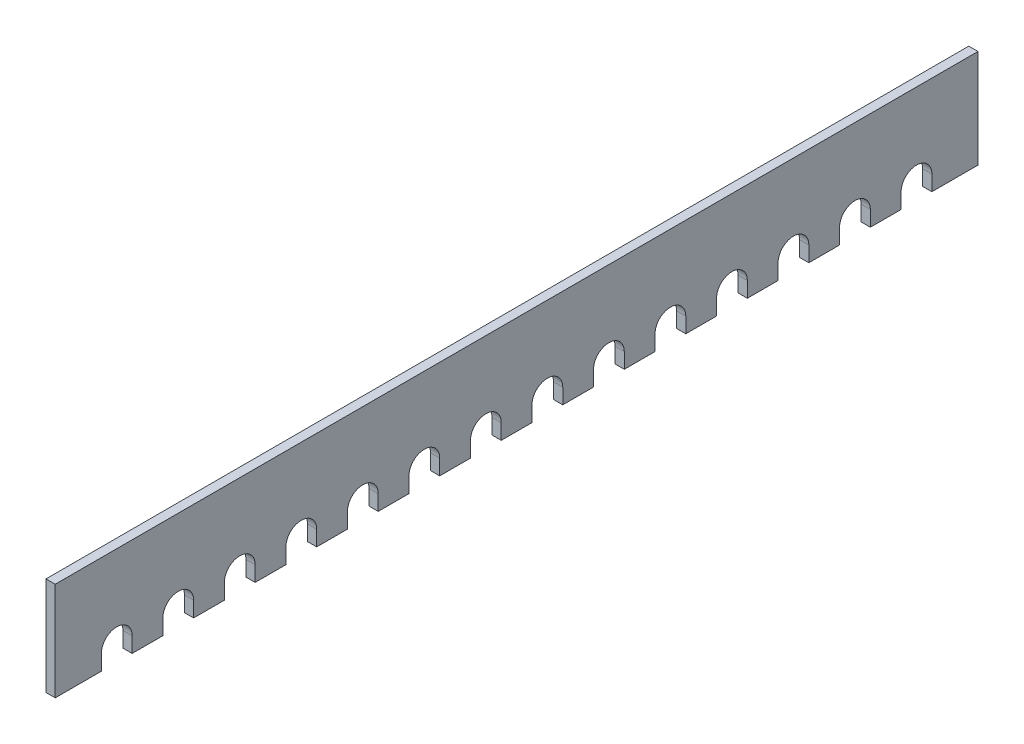
SolidWorks part; units mm, degrees
material "Plain Carbon Steel"
ref_plane "Front Plane" through (0, 0, 0) normal (0, 0, 1) x (1, 0, 0)
ref_plane "Top Plane" through (0, 0, 0) normal (0, 1, 0) x (1, 0, 0)
ref_plane "Right Plane" through (0, 0, 0) normal (1, 0, 0) x (0, 0, -1)
sketch "Sketch1" plane through (0, 0, 0) normal (0, 0, 1) x (1, 0, 0)
  line L1 (0, 0) -> (0, -32)
  dimension "D1" = 32
extrude "Extrude-Thin1" add sketch "Sketch1" along normal blind 300 thin
sketch "Sketch2" plane through (0, 0, 0) normal (1, 0, 0) x (0, 0, -1)
  line L0 (-300, -32) -> (0, -32) construction
  line L1 (-300, 0) -> (-300, -32) construction
  line L2 (-275, -27) -> (-275, -32)
  line L3 (-275, -32) -> (-285, -32)
  line L4 (-285, -32) -> (-285, -27)
  arc A0 (-275, -27) -> (-285, -27) centre (-280, -27) ccw
  dimension "D1" = 10
  dimension "D2" = 5
  dimension "D3" = 20
extrude "Cut-Extrude1" cut sketch "Sketch2" against normal through all
pattern_linear "LPattern1" count 14 spacing 20 along (0, 0, -1) of "Cut-Extrude1"
